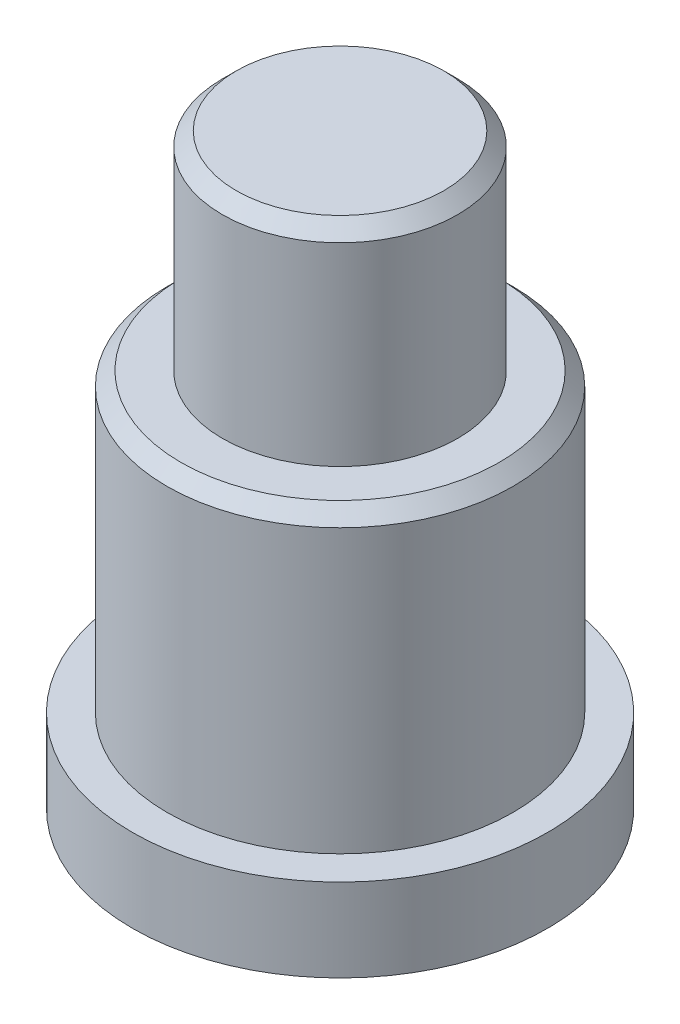
SolidWorks part; units mm, degrees
material "20#"
ref_plane "Front Plane" through (0, 0, 0) normal (0, 0, 1) x (1, 0, 0)
ref_plane "Top Plane" through (0, 0, 0) normal (0, 1, 0) x (1, 0, 0)
ref_plane "Right Plane" through (0, 0, 0) normal (1, 0, 0) x (0, 0, -1)
sketch "Sketch1" plane through (0, 0, 0) normal (0, 0, 1) x (1, 0, 0)
  line L0 (-99.0674, -10.1618) -> (-100.3174, -10.1618)
  line L1 (77.1826, -10.1618) -> (-167.8174, -10.1618) construction
  line L2 (-100.3174, -10.1618) -> (-100.3174, -13.1618)
  line L3 (-100.3174, -13.1618) -> (-92.8174, -13.1618)
  line L4 (-99.0674, -10.1618) -> (-99.0674, 0.5382)
  line L7 (-92.8174, 8.1026) -> (-92.8174, -13.1618) construction
  line L10 (-99.0674, 0.5382) -> (-97.0674, 0.5382)
  line L11 (-97.0674, 0.5382) -> (-97.0674, 8.0382)
  line L12 (87.1826, 1.0382) -> (-177.8174, 1.0382) construction
  line L13 (-88.6294, 8.1026) -> (-97.0054, 8.1026) construction
  line L14 (-97.0674, 8.0382) -> (-92.8174, 8.0382)
  line L16 (-92.8174, -13.1618) -> (-92.8174, 8.0382)
  dimension "D1" = 0.5
  dimension "D2" = 7.5
  dimension "D3" = 8.5
  dimension "D4" = 3
  dimension "D5" = 15
revolve "Revolve1" add sketch "Sketch1" angle 360 about L7
chamfer "Chamfer1" distance 0.5 angle 45 2 edges at (-92.8174, 0.5382, 6.25) (-92.8174, 8.0382, 4.25)
